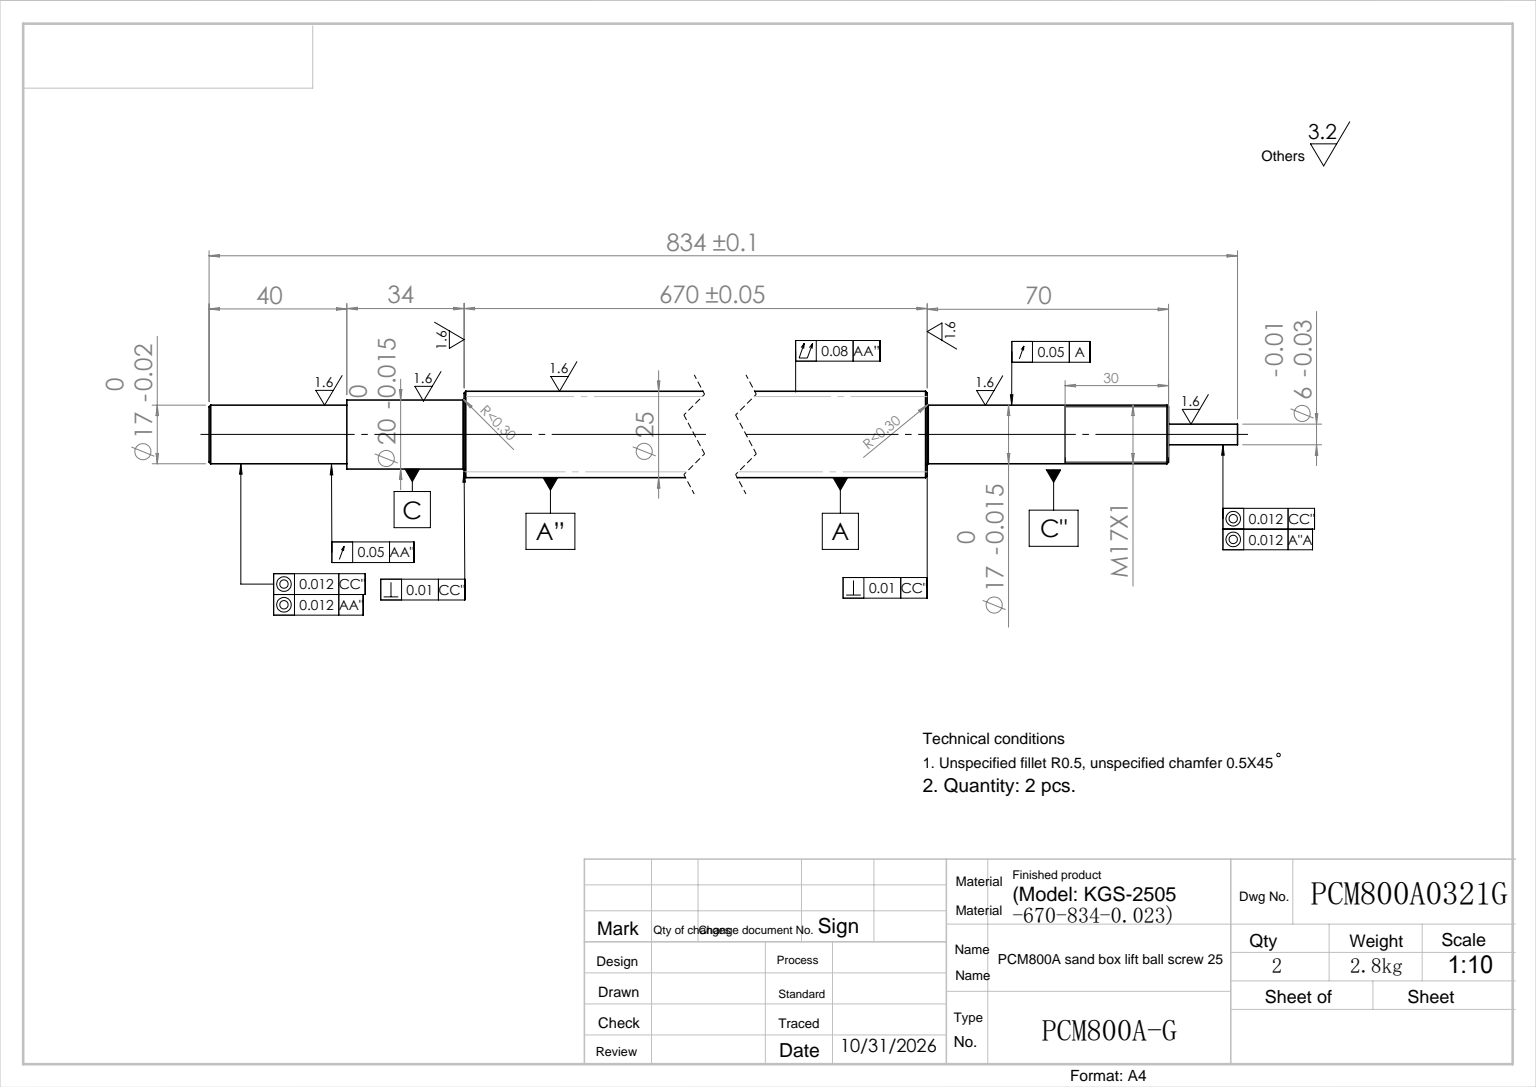
from build123d import *

# Parameters (mm, degrees)
SKETCH_1_R      = 8.5
EXTRUDE_1_DEPTH = 70
SKETCH_2_R      = 12.5
EXTRUDE_2_DEPTH = 670
SKETCH_3_R      = 10
EXTRUDE_3_DEPTH = 34
SKETCH_4_R      = 8.5
EXTRUDE_4_DEPTH = 40
CHAMFER_1_SIZE  = 0.5
FILLET_1_R      = 0.3
FILLET_2_R      = 0.3
SKETCH_5_R      = 3
EXTRUDE_5_DEPTH = 20


with BuildPart() as part:
    # 草图1 → 拉伸1 (new body)
    with BuildSketch(Plane(origin=(0, 0, 0), x_dir=(1, 0, 0), z_dir=(0, 1, 0))):
        with Locations(Location((0, 0, 0), (0, 0, 270))):
            Circle(SKETCH_1_R)
    extrude(amount=EXTRUDE_1_DEPTH)

    # 草图2 → 拉伸2 (add)
    with BuildSketch(Plane(origin=(0, 70, 0), x_dir=(-1, 0, 0), z_dir=(0, 1, 0))):
        with Locations(Location((0, 0, 0), (0, 0, 90))):
            Circle(SKETCH_2_R)
    extrude(amount=EXTRUDE_2_DEPTH)

    # 草图3 → 拉伸3 (add)
    with BuildSketch(Plane(origin=(0, 740, 0), x_dir=(-1, 0, 0), z_dir=(0, 1, 0))):
        with Locations(Location((0, 0, 0), (0, 0, 90))):
            Circle(SKETCH_3_R)
    extrude(amount=EXTRUDE_3_DEPTH)

    # 草图4 → 拉伸4 (add)
    with BuildSketch(Plane(origin=(0, 774, 0), x_dir=(-1, 0, 0), z_dir=(0, 1, 0))):
        with Locations(Location((0, 0, 0), (0, 0, 90))):
            Circle(SKETCH_4_R)
    extrude(amount=EXTRUDE_4_DEPTH)

    # 倒角1
    chamfer_1_edges = [part.edges().sort_by_distance(p)[0] for p in [
        (0, 814, -8.5),
        (0, 0, -8.5),
        (0, 70, -12.5),
        (0, 740, -12.5),
    ]]
    chamfer(chamfer_1_edges, length=CHAMFER_1_SIZE)

    # 圆角1
    fillet_1_edges = [part.edges().sort_by_distance(p)[0] for p in [
        (0, 70, -8.5),
    ]]
    fillet(fillet_1_edges, radius=FILLET_1_R)

    # 圆角2
    fillet_2_edges = [part.edges().sort_by_distance(p)[0] for p in [
        (0, 740, -10),
    ]]
    fillet(fillet_2_edges, radius=FILLET_2_R)

    # 草图5 → 拉伸5 (add)
    with BuildSketch(Plane.XZ):
        with Locations(Location((0, 0, 0), (0, 0, 90))):
            Circle(SKETCH_5_R)
    extrude(amount=EXTRUDE_5_DEPTH)


solid = part.part
